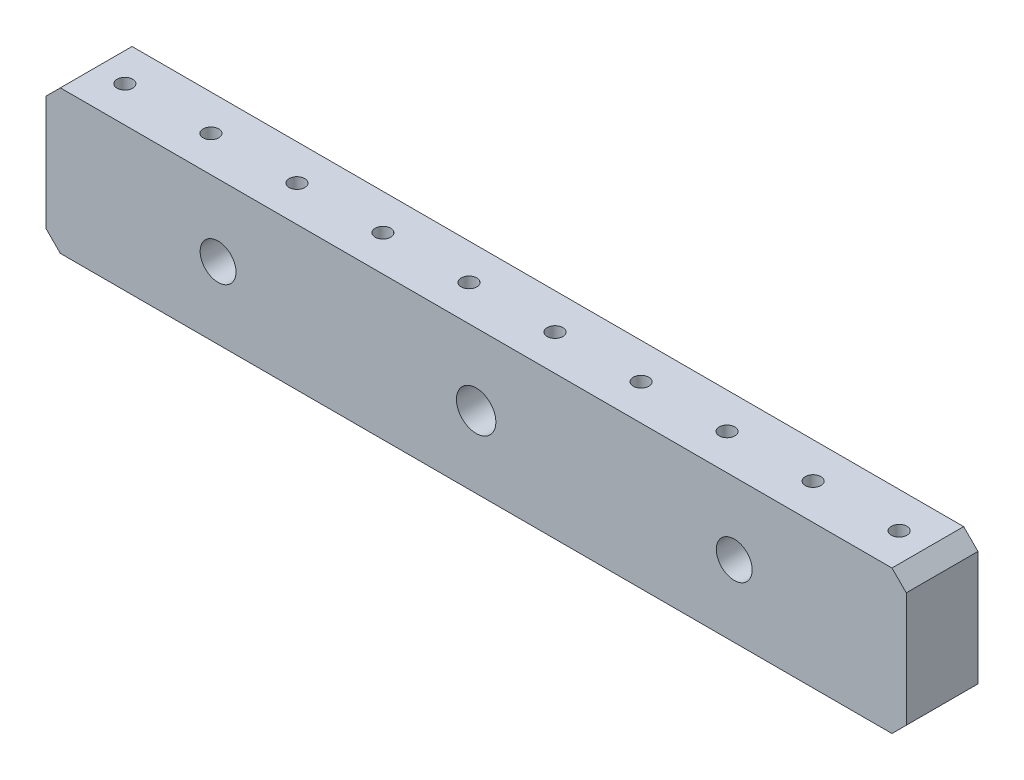
SolidWorks part; units mm, degrees
material "SUS304"
ref_plane "前视基准面" through (0, 0, 0) normal (0, 0, 1) x (1, 0, 0)
ref_plane "上视基准面" through (0, 0, 0) normal (0, 1, 0) x (1, 0, 0)
ref_plane "右视基准面" through (0, 0, 0) normal (1, 0, 0) x (0, 0, -1)
sketch "草图1" plane through (0, 0, 0) normal (0, 1, 0) x (1, 0, 0)
  line L1 (-60, 5) -> (60, 5)
  line L2 (-60, 5) -> (-60, -5)
  line L3 (-60, -5) -> (60, -5)
  line L4 (60, 5) -> (60, -5)
  line L5 (-60, 5) -> (60, -5) construction
  line L6 (-60, -5) -> (60, 5) construction
  point P0 (0, 0)
  dimension "D1" = 120
  dimension "D2" = 10
extrude "凸台-拉伸1" add sketch "草图1" along normal blind 20
sketch "草图2" plane through (0, 20, 0) normal (0, 1, 0) x (1, 0, 0)
  line L0 (60, 5) -> (-60, 5) construction
  line L1 (-60, 5) -> (-60, -5) construction
  circle A0 centre (-54, 0) radius 1.09
  dimension "D1" = 2.18
  dimension "D2" = 5
  dimension "D3" = 6
extrude "切除-拉伸1" cut sketch "草图2" against normal blind 3
sketch "草图4" plane through (0, 17, 0) normal (0, 1, 0) x (1, 0, 0)
  circle A0 centre (-54, 0) radius 0.825
  dimension "D1" = 1.65
extrude "切除-拉伸2" cut sketch "草图4" against normal blind 30
pattern_linear "阵列(线性)1" count 10 spacing 12 along (1, 0, 0) of "切除-拉伸2", "切除-拉伸1"
chamfer "倒角1" distance 2 angle 45 4 edges at (60, 20, 0) (60, 0, 0) (-60, 20, 0) (-60, 0, 0)
hole_wizard "大小mm 暗销孔1" positions "草图6" profile "草图7" hole size "Ø5.0" standard "GB"
sketch "草图6" plane through (0, 0, 5) normal (0, 0, 1) x (1, 0, 0)
  line L0 (-58, 0) -> (58, 0) construction
  line L1 (60, 18) -> (60, 2) construction
  line L2 (-60, 18) -> (-60, 2) construction
  point P0 (36, 10)
  point P2 (-36, 10)
  dimension "D1" = 10
  dimension "D2" = 24
  dimension "D3" = 24
sketch "草图7" plane through (36, 10, 5) normal (1, 0, 0) x (0, -1, 0)
  line L0 (0, 0) -> (0, 16.5022)
  line L1 (0, 16.5022) -> (2.5, 15)
  line L2 (2.5, 15) -> (2.5, 0)
  line L5 (2.5, 0) -> (0, 0)
  line L10 (0, 16.5022) -> (-2.5, 15) construction
  line L11 (0, -6.35) -> (0, 107.95) construction
  dimension "孔直径" = 5
  dimension "孔深度" = 15
  dimension "导头角度" = 118
hole_wizard "M5 间隙孔1" positions "草图8" profile "草图9" hole size "M5" standard "GB"
sketch "草图8" plane through (0, 0, 5) normal (0, 0, 1) x (1, 0, 0)
  line L0 (-58, 20) -> (58, 20) construction
  line L1 (-60, 18) -> (-60, 2) construction
  point P0 (0, 10)
  dimension "D1" = 10
  dimension "D2" = 60
sketch "草图9" plane through (0, 10, 5) normal (1, 0, 0) x (0, -1, 0)
  line L0 (0, 0) -> (0, 16.6524)
  line L1 (0, 16.6524) -> (2.75, 15)
  line L2 (2.75, 15) -> (2.75, 0)
  line L5 (2.75, 0) -> (0, 0)
  line L10 (0, 16.6524) -> (-2.75, 15) construction
  line L11 (0, -6.35) -> (0, 107.95) construction
  dimension "孔直径" = 5.5
  dimension "孔深度" = 15
  dimension "导头角度" = 118
